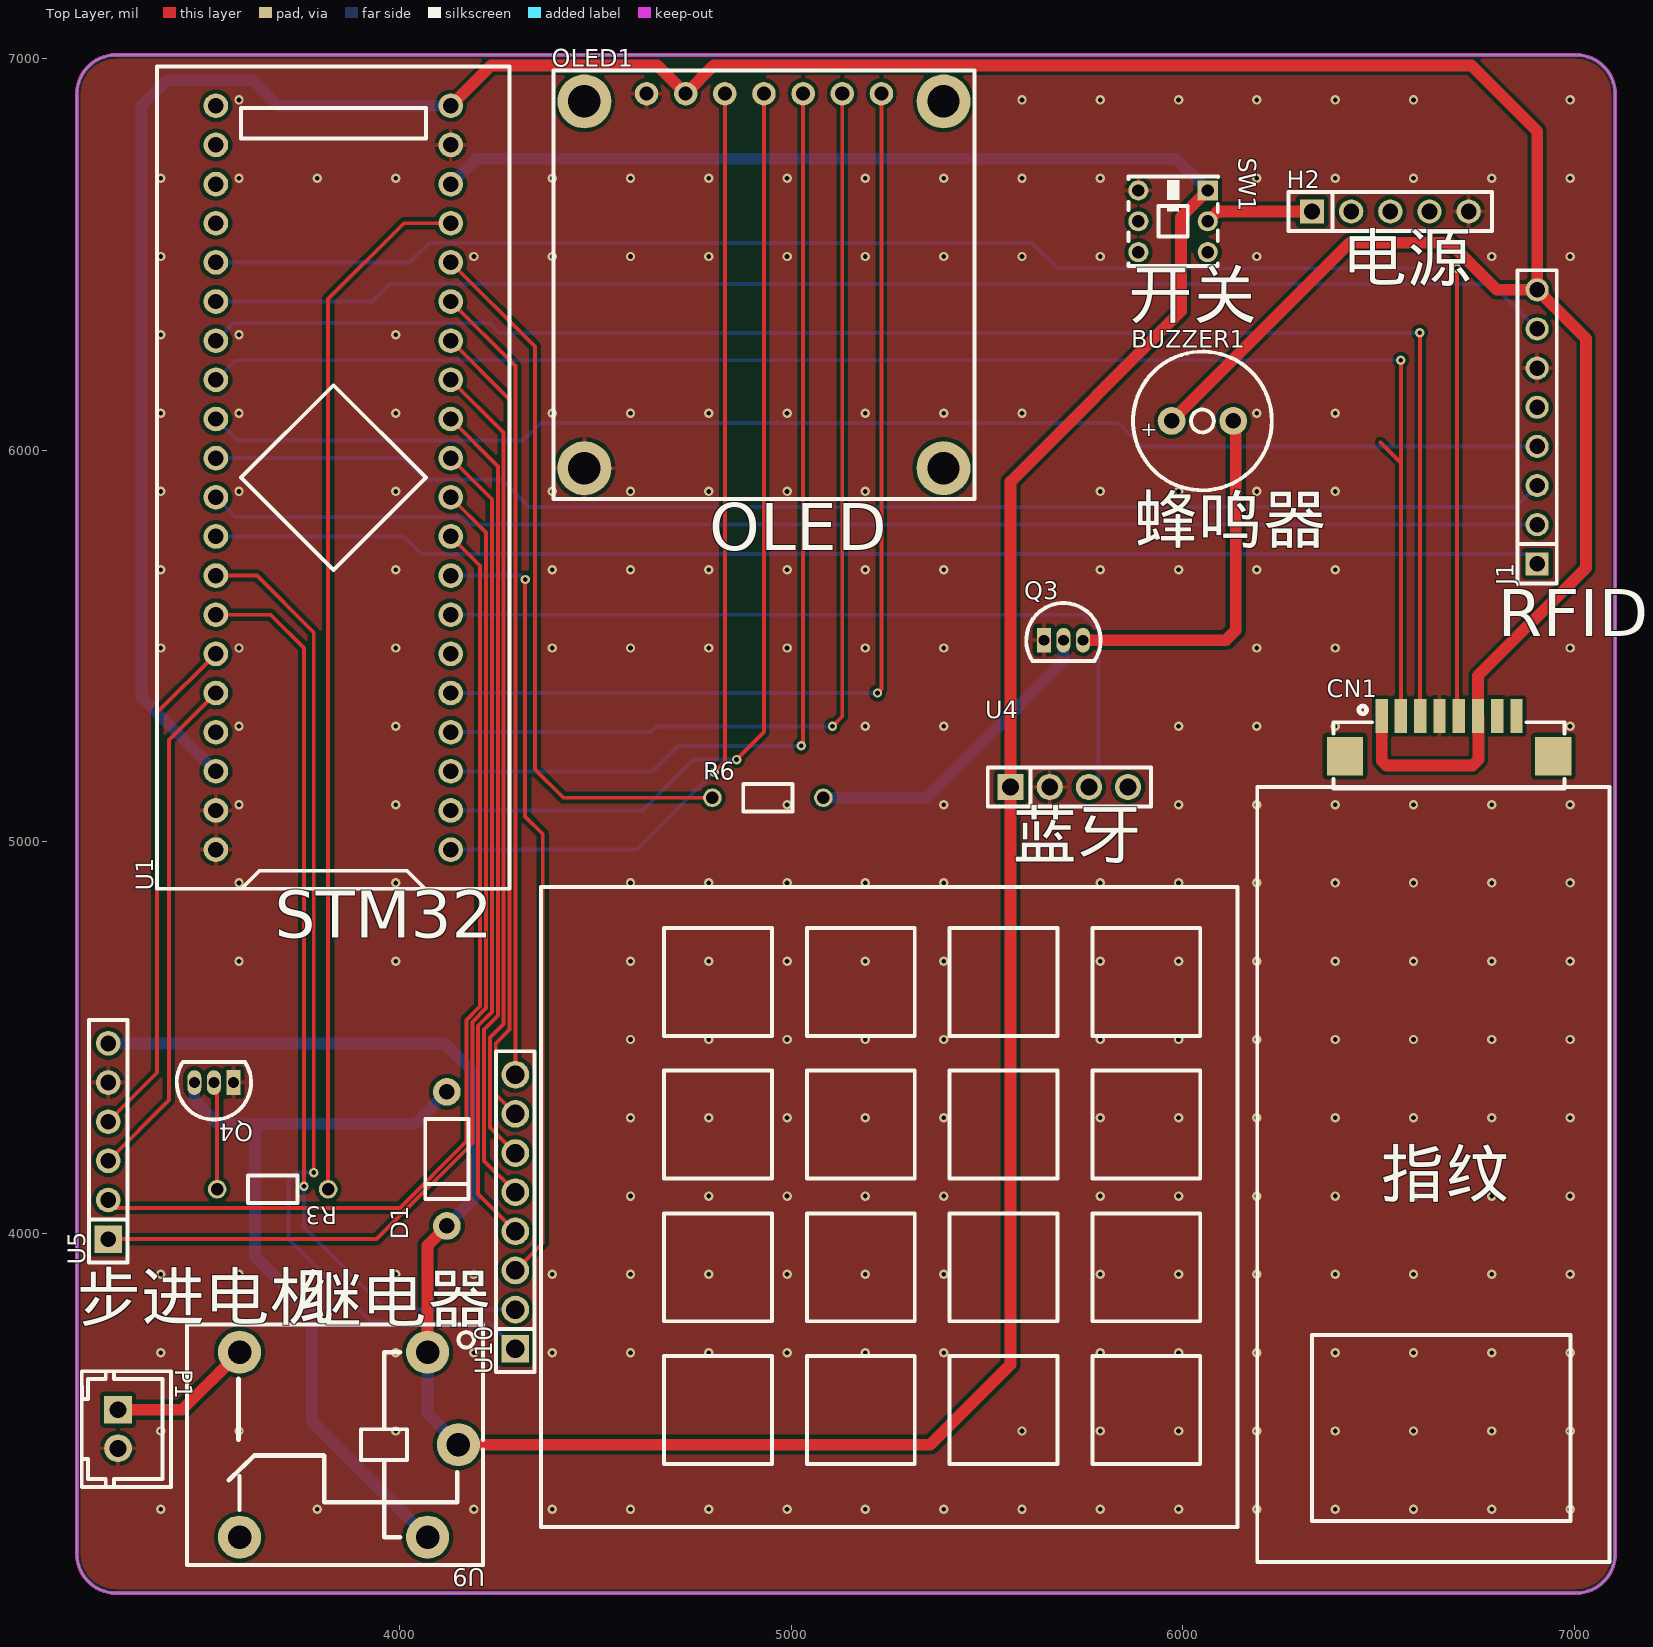
[diagram p0: Top Layer view]
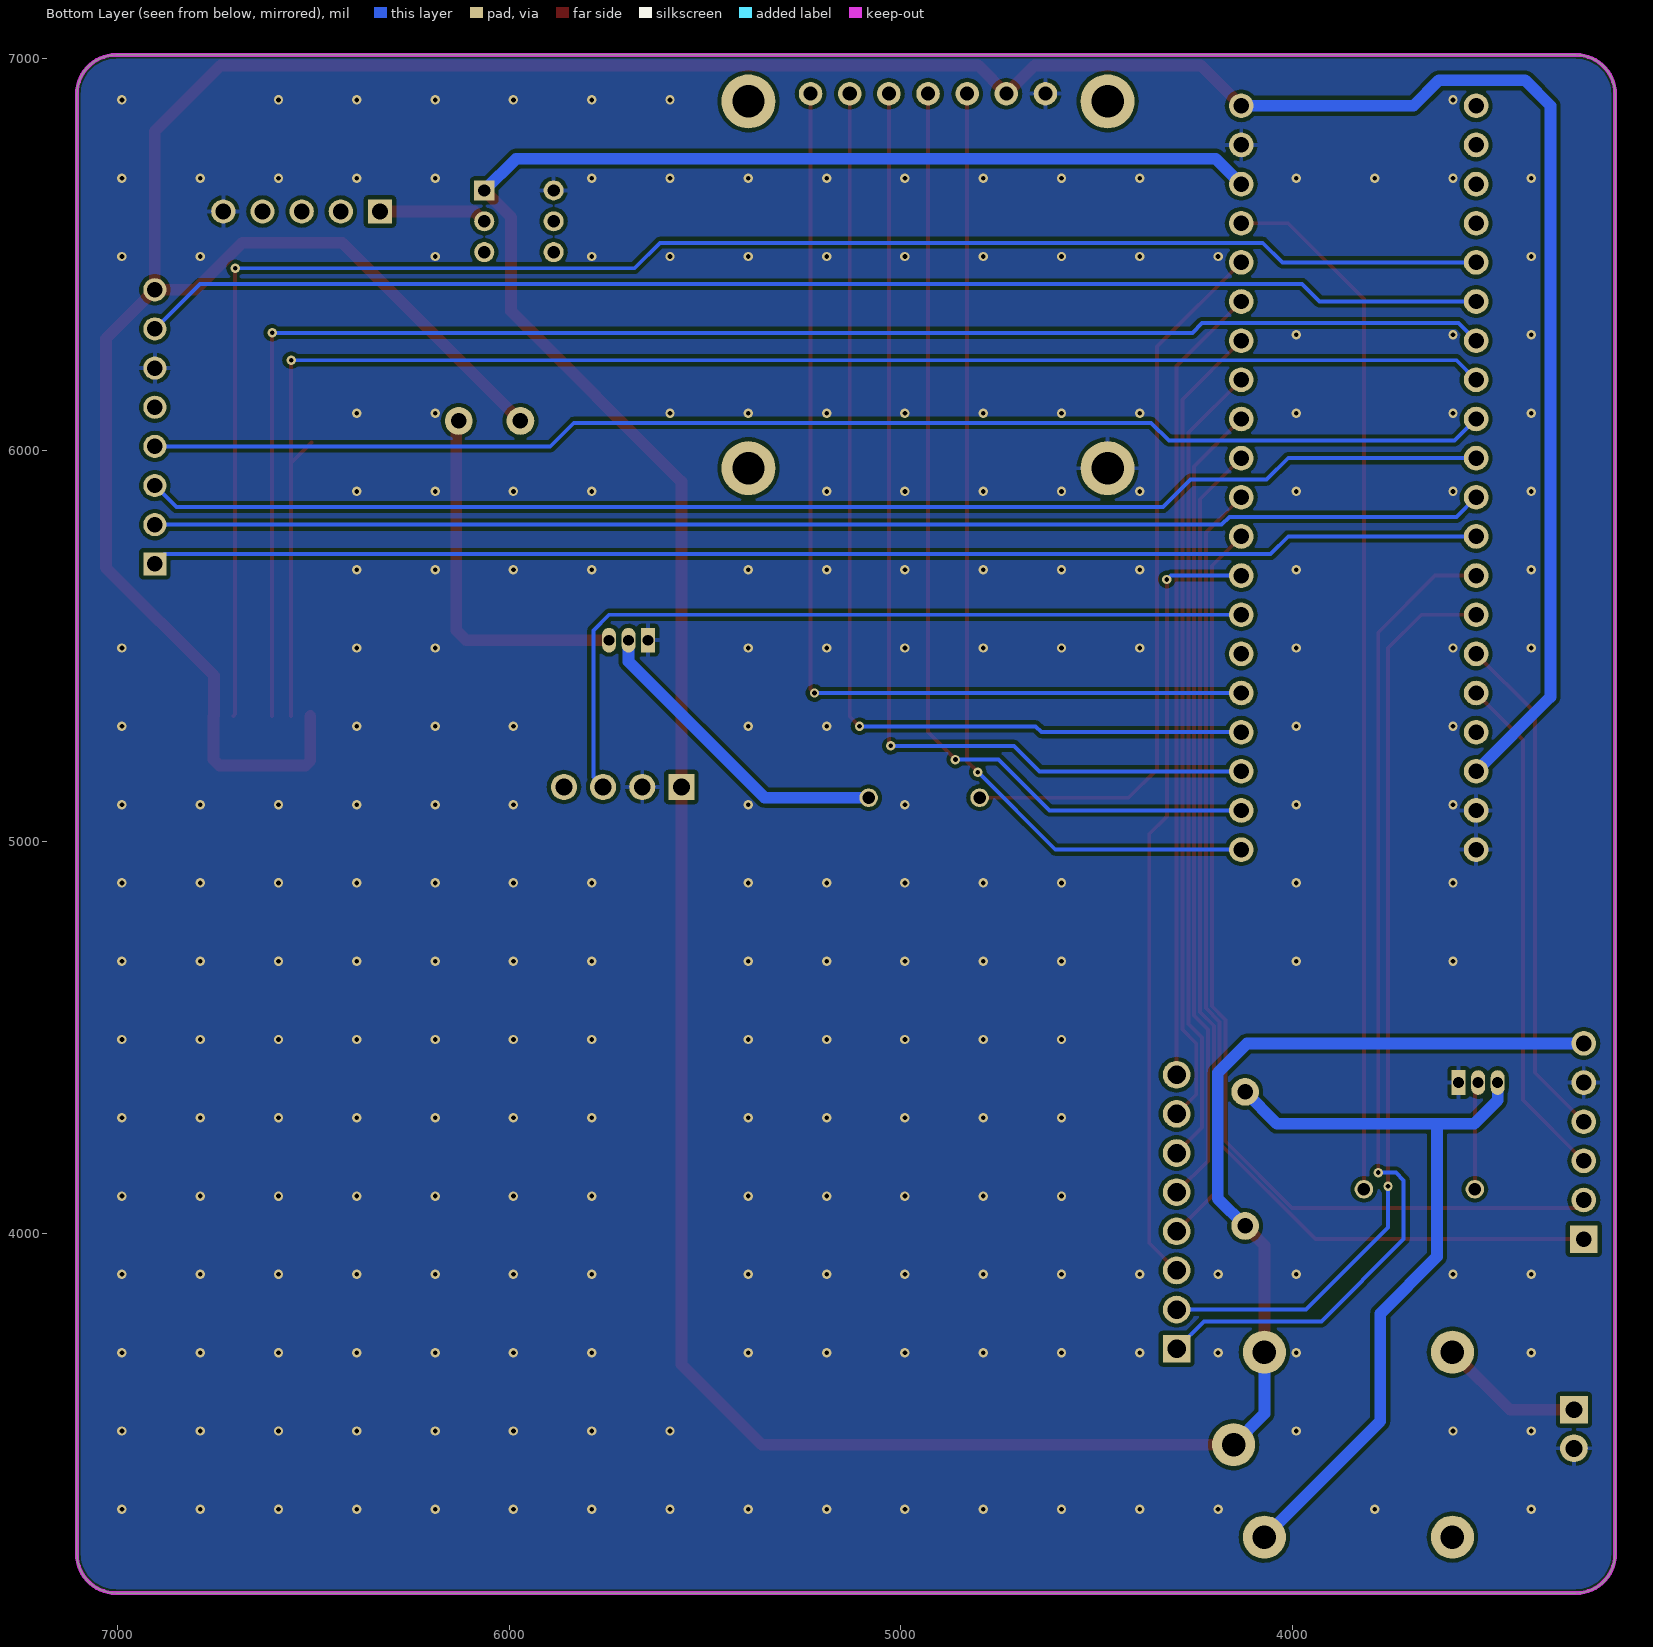
[diagram p1: Bottom Layer view, seen from below]
# Altium PCB MISC51826.pcbdoc
Units mil, origin at the board's own origin, x right, y up, seen from the top; angles counter-clockwise.
Board outline 3929.13 x 3929.13 mil, 2 copper layers (Top Layer, Bottom Layer), stack 62.206 mil thick; 17 components, 39 nets, 119 pads, 243 vias.

## Layer stack, top to bottom
Top Solder Mask Layer: solder mask 0.394, Dk 3.3
Top Layer: signal copper 1.379
Dielectric1: surface 59.449, FR4, Dk 4.5
Bottom Layer: signal copper 1.378
Bottom Solder Mask Layer: solder mask 0.394, Dk 3.3

## Board outline
3275,7010 ccw(c3275,6910) 3175,6910 3175,3180.87 ccw(c3275,3180.87) 3275,3080.87 7004.13,3080.87 ccw(c7004.13,3180.87) 7104.13,3180.87 7104.13,6910 ccw(c7004.13,6910) 7004.13,7010

## Design rules (kind name [scope] priority, off if disabled: settings)
BoardOutlineClearance copperThickness2oz_1 [All] p2 off: genericclearance=7.99 ignorepadtopadclearanceinfootprint=FALSE except(0: Arc-SplitContinuation Track-SplitContinuation SMDPad-SplitContinuation THPad-SplitContinuation Via-SplitContinuation Fill-SplitContinuation Region-SplitContinuation Poly-SplitContinuation Text-SplitContinuation Hole-SplitContinuation; 5.98: Arc-CutoutEdge SMDPad-CutoutEdge THPad-CutoutEdge Via-CutoutEdge Fill-CutoutEdge Region-CutoutEdge Text-CutoutEdge; 6.93: Hole-OutlineEdge Hole-CutoutEdge; 10: Poly-OutlineEdge Poly-CutoutEdge; 11.81: Arc-OutlineEdge Track-OutlineEdge SMDPad-OutlineEdge THPad-OutlineEdge Via-OutlineEdge Fill-OutlineEdge Region-OutlineEdge Text-OutlineEdge Track-CutoutEdge)
BoardOutlineClearance copperThickness1oz_1 [All] p4: genericclearance=4.02 ignorepadtopadclearanceinfootprint=FALSE except(0: Arc-SplitContinuation Track-SplitContinuation SMDPad-SplitContinuation THPad-SplitContinuation Via-SplitContinuation Fill-SplitContinuation Region-SplitContinuation Poly-SplitContinuation Text-SplitContinuation Hole-SplitContinuation; 6: SMDPad-CutoutEdge THPad-CutoutEdge Via-CutoutEdge Fill-CutoutEdge Region-CutoutEdge Text-CutoutEdge; 6.93: Hole-OutlineEdge Hole-CutoutEdge; 10: Poly-OutlineEdge Poly-CutoutEdge; 11.8: Arc-OutlineEdge Track-OutlineEdge SMDPad-OutlineEdge THPad-OutlineEdge Via-OutlineEdge Fill-OutlineEdge Region-OutlineEdge Text-OutlineEdge; 11.81: Arc-CutoutEdge Track-CutoutEdge)
Clearance copperThickness2oz [All] p1 off: gap=7.99 ignorepadtopadclearanceinfootprint=FALSE except(5.98: SMDPad-Track SMDPad-SMDPad THPad-Track SMDPad-THPad THPad-THPad Track-Via SMDPad-Via THPad-Via Via-Via Fill-Track Region-Track Fill-SMDPad Region-SMDPad Fill-THPad Region-THPad Fill-Via Region-Via Fill-Fill Fill-Region Region-Region Arc-Track Arc-SMDPad Arc-THPad Arc-Via Fill-Arc Region-Arc Arc-Arc Text-Track SMDPad-Text Text-THPad Text-Via Fill-Text Region-Text Arc-Text Text-Text; 6.93: Hole-Track Hole-SMDPad Hole-THPad Hole-Via Fill-Hole Region-Hole Hole-Arc Hole-Text; 10: Poly-Track Poly-SMDPad Poly-THPad Poly-Via Poly-Fill Poly-Region Poly-Poly Poly-Arc Poly-Text Poly-Hole)
Clearance copperThickness1oz [All] p3: gap=4.02 ignorepadtopadclearanceinfootprint=FALSE except(5.98: SMDPad-Track SMDPad-SMDPad THPad-Track SMDPad-THPad THPad-THPad Track-Via SMDPad-Via THPad-Via Via-Via Fill-Track Region-Track Fill-SMDPad Region-SMDPad Fill-THPad Region-THPad Fill-Via Region-Via Fill-Fill Fill-Region Region-Region; 6: Arc-Track Arc-SMDPad Arc-THPad Arc-Via Fill-Arc Region-Arc Arc-Arc Text-Track SMDPad-Text Text-THPad Text-Via Fill-Text Region-Text Arc-Text Text-Text; 6.93: Hole-Track Hole-SMDPad Hole-THPad Hole-Via Fill-Hole Region-Hole Hole-Arc Hole-Text; 10: Poly-Track Poly-SMDPad Poly-THPad Poly-Via Poly-Fill Poly-Region Poly-Poly Poly-Arc Poly-Text Poly-Hole)
DiffPairsRouting differentialPair [All] p1: maxlimit=6 minlimit=6 mostfreqgap=6 toplayer_minwidth=5 toplayer_prefwidth=10 toplayer_maxwidth=100 toplayer_mingap=6 toplayer_prefgap=6 toplayer_maxgap=6 bottomlayer_minwidth=5 bottomlayer_prefwidth=10 bottomlayer_maxwidth=100 bottomlayer_mingap=6 bottomlayer_prefgap=6 bottomlayer_maxgap=6 maxuncoupledlength=10
HoleToHoleClearance otherClearance [All] p1: gap=11.81 allowstackedmicrovias=TRUE
Length netLength [All] p1: minlimit=0 maxlimit=0
MatchedLengths netLengthTolerance [All] p1: tolerance=1000
PasteMaskExpansion pasteMaskExpansion [All] p1: expansion=0
PlaneConnect innerPlane [All] p1: planeconnectstyle=Relief reliefexpansion=20 reliefentries=4 reliefconductorwidth=10 reliefairgap=10
PolygonConnect copperRegion [(InNet('GND'))] p1: connectstyle=Relief reliefconductorwidth=10 reliefentries=4 polygonreliefangle="90 Angle" airgapwidth=10 via.connectstyle=Relief via.reliefconductorwidth=10 via.reliefentries=4 via.polygonreliefangle="90 Angle" via.airgapwidth=10
RoutingVias viaSize [All] p1: holewidth=12.01 width=24.02 viastyle="Through Hole" minholewidth=11.81 minwidth=19.68 maxholewidth=248.03 maxwidth=393.7
SolderMaskExpansion solderMaskExpansion [IsVia] p1: expansion=-1000 istentingtop=TRUE
SolderMaskExpansion solderMaskExpansion [All] p2: expansion=2 istentingtop=FALSE
Width copperThickness2oz_2 [All] p1 off: maxlimit=100 minlimit=8 preferedwidth=10
Width copperThickness1oz_2 [All] p2: maxlimit=100 minlimit=5 preferedwidth=10

## Components (designator, comment, footprint, x,y, rotation, side; value= is the part's Value field where it differs from the comment)
BUZZER1 "2.7kHz" BUZ-TH_BD9.0-P4.00-D0.6-FD 6050,6075 r0 top
CN1 "AS608" AS608 6680,5270 r0 top
D1 "" DO_1N4007 4120,4190 r90 top
H2 "" HDR-TH_5P-P2.54-V-F 6530,6610 r0 top
J1 "" HDR-TH_8P-P2.54-V-M 6905,6060 r90 top
OLED1 "" 0.96OLED 4930,6970 r0 top
P1 "WAFER-XH254Z-2A" CONN-TH_2P-P2.50_XH-2A_3045048 3280,3500 r270 top
Q3 "" S8050_TO_92 5695,5515 r0 top
Q4 "" S8050_TO_92 3525,4385 r180 top
R3 "1K" Res_1/8W 3675,4115 r180 top
R6 "1K" Res_1/8W 4940,5110 r0 top
SW1 "5.8 WSPT" SW-TH_6P-L5.8-W5.8-P2.00-LS4.5-TL_K8-5851E-L1 5975,6585 r270 top
U1 "LCKFB-DKX-STM32F103C8T6" CONN-TH_L53.3-W22.9_STM32F103C8T6-CARD 3830,5930 r90 top
U4 "" HDR-TH_4P-P2.54-V-F 5710,5140 r0 top
U5 "" HDR-TH_6P-P2.54-V-F 3255,4235 r90 top
U9 "SRD-12VDC-SL-C" RELAY-TH_SRD-XXVDC-XL-C 3870,3460 r180 top
U10 "" HDR-TH_8P-P2.54-V-F-1 4295,4055 r90 top

## Footprints (in the part's own frame and the unit in brackets; to place one, negate y for a bottom-side part, rotate by r counter-clockwise, add the part's x,y. Pads: shape width x height; smd on the part's side, far side on the other; paste and mask are expansions set on the pad)
0.96OLED [mm]
  round 3.5 hole 2.1: 0(-11.65,-2) 1(-11.65,-25.8) 8(11.65,-2) 9(11.65,-25.8)
  round 1.524 hole 0.914: 1(-7.62,-1.5) 2(-5.08,-1.5) 3(-2.54,-1.5) 4(0,-1.5) 5(2.54,-1.5) 6(5.08,-1.5) 7(7.62,-1.5)
  silkscreen extent -13.65,-27.8 13.65,0
AS608 [mm]
  rect 0.8x2.2 smd paste+0 mask+0.05: 1(-4.375,1.3) 2(-3.125,1.3) 3(-1.875,1.3) 4(-0.625,1.3) 5(0.625,1.3) 6(1.875,1.3) 7(3.125,1.3) 8(4.375,1.3)
  rect 2.35x2.5 smd paste+0 mask+0.05: 9(-6.755,-1.3) 10(6.755,-1.3)
  silkscreen extent -7.5,-3.4 7.5,1.95
BUZ-TH_BD9.0-P4.00-D0.6-FD [mm]
  round 1.8 hole 1: 1(-2,0) 2(2,0)
  silkscreen extent -4.5,-4.5 4.5,4.5
CONN-TH_2P-P2.50_XH-2A_3045048 [mm]
  rect 1.8x1.8 hole 1.1 paste+0 mask+0.05: 1(-1.25,0)
  round 1.8 hole 1.1 paste+0 mask+0.05: 2(1.25,0)
  silkscreen extent -3.75,-2.35 3.75,3.45
CONN-TH_L53.3-W22.9_STM32F103C8T6-CARD [mm]
  round 1.6 hole 1: 1(-24.13,-7.62) 2(-21.59,-7.62) 3(-19.05,-7.62) 4(-16.51,-7.62) 5(-13.97,-7.62) 6(-11.43,-7.62) 7(-8.89,-7.62) 8(-6.35,-7.62) 9(-3.81,-7.62) 10(-1.27,-7.62) 11(1.27,-7.62) 12(3.81,-7.62) 13(6.35,-7.62) 14(8.89,-7.62) 15(11.43,-7.62) 16(13.97,-7.62) 17(16.51,-7.62) 18(19.05,-7.62) 19(21.59,-7.62) 20(24.13,-7.62) 21(24.13,7.62) 22(21.59,7.62) 23(19.05,7.62) 24(16.51,7.62) 25(13.97,7.62) 26(11.43,7.62) 27(8.89,7.62) 28(6.35,7.62) 29(3.81,7.62) 30(1.27,7.62) 31(-1.27,7.62) 32(-3.81,7.62) 33(-6.35,7.62) 34(-8.89,7.62) 35(-11.43,7.62) 36(-13.97,7.62) 37(-16.51,7.62) 38(-19.05,7.62) 39(-21.59,7.62) 40(-24.13,7.62)
  silkscreen extent -26.67,-11.43 26.67,11.43
DO_1N4007 [mm]
  round 1.8 hole 1 paste+0 mask+0.051: 1(-4.35,0) 2(4.35,0)
  silkscreen extent -2.6,-1.4 2.6,1.4
HDR-TH_4P-P2.54-V-F [mm]
  rect 1.7x1.7 hole 1.1: 1(-3.81,0)
  round 1.7 hole 1.1: 2(-1.27,0) 3(1.27,0) 4(3.81,0)
  silkscreen extent -5.29,-1.27 5.29,1.27
HDR-TH_5P-P2.54-V-F [mil]
  rect 62x62 hole 40.16: 1(-200,0)
  round 62 hole 40.16: 2(-100,0) 3(0,0) 4(100,0) 5(200,0)
  silkscreen extent -260,-50 260,50
HDR-TH_6P-P2.54-V-F [mm]
  rect 1.8x1.8 hole 1.02: 1(-6.35,0)
  round 1.6 hole 1.02: 2(-3.81,0) 3(-1.27,0) 4(1.27,0) 5(3.81,0) 6(6.35,0)
  silkscreen extent -7.87,-1.25 7.87,1.25
HDR-TH_8P-P2.54-V-F-1 [mm]
  rect 1.8x1.8 hole 1.2: 1(-8.89,0)
  round 1.8 hole 1.2: 2(-6.35,0) 3(-3.81,0) 4(-1.27,0) 5(1.27,0) 6(3.81,0) 7(6.35,0) 8(8.89,0)
  silkscreen extent -10.41,-1.25 10.41,1.25
HDR-TH_8P-P2.54-V-M [mm]
  rect 1.5x1.5 hole 1: 1(-8.89,0)
  round 1.5 hole 1: 2(-6.35,0) 3(-3.81,0) 4(-1.27,0) 5(1.27,0) 6(3.81,0) 7(6.35,0) 8(8.89,0)
  silkscreen extent -10.16,-1.27 10.16,1.27
RELAY-TH_SRD-XXVDC-XL-C [mil]
  round 110 hole 60: 1(-200.79,-236.22) 2(279.53,-236.2) 3(279.53,236.2) 4(-200.79,236.22) 5(-279.53,0)
  silkscreen extent -342,-307 413,307
Res_1/8W [mil]
  round 47.2 hole 31.5 paste+0 mask+2: 1(-141.7,2.48) 2(141.7,2.48)
  silkscreen extent -63,-33 63,38
S8050_TO_92 [mil]
  rect 35.4x63 hole 27.6 paste+0 mask+2: 1(-50,0)
  oval 35.4x63 hole 27.6 paste+0 mask+2: 2(0,0) 3(50,0)
  silkscreen extent -95,-53 95,95
SW-TH_6P-L5.8-W5.8-P2.00-LS4.5-TL_K8-5851E-L1 [mm]
  rect 1.3x1.3 hole 0.8 paste+0 mask+0.05: 1(-2,2.25)
  round 1.3 hole 0.8 paste+0 mask+0.05: 2(0,2.25) 3(2,2.25) 4(-2,-2.25) 5(0,-2.25) 6(2,-2.25)
  silkscreen extent -2.9,-2.9 2.9,2.92

## Via types
v1: diameter 24.02, hole 12, Top Layer to Bottom Layer, 243 vias

## Nets (pads, with @x,y where several pads share a name; then routed paths per layer and width w, separated by ;. In a path a pad name is that pad's centre, name@x,y a point inside that pad or via, vN(x,y) a via of type N, cw(c..) or ccw(c..) an arc to the next point about the centre after c; other vN are vias at no path point)
$1N3: Q4.2 R3.2 | length 275.9
  Top Layer w10: Q4.2 3533.3,4376.7 R3.2
$1N6: D1.2 Q4.3 U9.4 | length 1977.3
  Bottom Layer w30: Q4.3 3475,4340 3535,4280 4038.74,4280 D1.2 ; 3630,4270 3630,3940 3775,3795 3775,3519.57 U9.4
$1N8: P1.1 U9.2 | length 371.4
  Top Layer w30: P1.1 3443.48,3549.21 U9.2
$1N34: H2.1 SW1.2 | length 276.8
  Top Layer w30: SW1.2 6088.59,6610 H2.1
$1N53: Q3.2 R6.2 | length 812.2
  Bottom Layer w30: R6.2 5347.48,5112.48 5695,5460 Q3.2
$1N55: BUZZER1.2 Q3.3 | length 937.9
  Top Layer w30: Q3.3 6110,5515 6135,5540 6135,6068.74 BUZZER1.2
$1N71: U1.37
+5V: D1.1 SW1.1 U1.18 U4.1 U5.6 U9.1 U9.5 | length 8694.9
  Top Layer w30: U9.1 4070.79,3969.53 D1.1 ; U9.5 5355,3460 5560,3665 U4.1 5560,5920 5995,6355 5995,6595.15 SW1.1
  Bottom Layer w30: U5.6 4115,4485 4190,4410 4190,4088.74 D1.1 ; U9.1 4070.79,3538.74 U9.5 ; U1.18 4195,6745 5982.32,6745 SW1.1
BEEP: R6.1 U1.16 | length 1867.4
  Top Layer w10: U1.16 4345,6265 4345,5185 4417.52,5112.48 R6.1
GND: CN1.4 H2.5 J1.6 OLED1.1 P1.2 Q3.1 Q4.1 SW1.4 U1.19 U1.39 U1.40 U4.2 U5.5
  other v1: 3389.1,3294.97 3789.1,3294.97 4189.1,3294.97 4389.1,3294.97 4589.1,3294.97 4789.1,3294.97 4989.1,3294.97 5189.1,3294.97 5389.1,3294.97 5589.1,3294.97 5789.1,3294.97 5989.1,3294.97 6189.1,3294.97 6389.1,3294.97 6589.1,3294.97 6789.1,3294.97 6989.1,3294.97 3389.1,3494.97 3589.1,3494.97 3989.1,3494.97 5589.1,3494.97 5789.1,3494.97 5989.1,3494.97 6189.1,3494.97 6389.1,3494.97 6589.1,3494.97 6789.1,3494.97 6989.1,3494.97 3389.1,3694.97 3989.1,3694.97 4189.1,3694.97 4389.1,3694.97 4589.1,3694.97 4789.1,3694.97 4989.1,3694.97 5189.1,3694.97 5389.1,3694.97 5789.1,3694.97 5989.1,3694.97 6189.1,3694.97 6389.1,3694.97 6589.1,3694.97 6789.1,3694.97 6989.1,3694.97 3389.1,3894.97 3589.1,3894.97 3989.1,3894.97 4189.1,3894.97 4389.1,3894.97 4589.1,3894.97 4789.1,3894.97 4989.1,3894.97 5189.1,3894.97 5389.1,3894.97 5789.1,3894.97 5989.1,3894.97 6189.1,3894.97 6389.1,3894.97 6589.1,3894.97 6789.1,3894.97 6989.1,3894.97 4589.1,4094.97 4789.1,4094.97 4989.1,4094.97 5189.1,4094.97 5389.1,4094.97 5789.1,4094.97 5989.1,4094.97 6189.1,4094.97 6389.1,4094.97 6589.1,4094.97 6789.1,4094.97 6989.1,4094.97 4589.1,4294.97 4789.1,4294.97 4989.1,4294.97 5189.1,4294.97 5389.1,4294.97 5789.1,4294.97 5989.1,4294.97 6189.1,4294.97 6389.1,4294.97 6589.1,4294.97 6789.1,4294.97 6989.1,4294.97 4589.1,4494.97 4789.1,4494.97 4989.1,4494.97 5189.1,4494.97 5389.1,4494.97 5789.1,4494.97 5989.1,4494.97 6189.1,4494.97 6389.1,4494.97 6589.1,4494.97 6789.1,4494.97 6989.1,4494.97 3589.1,4694.97 3989.1,4694.97 4589.1,4694.97 4789.1,4694.97 4989.1,4694.97 5189.1,4694.97 5389.1,4694.97 5789.1,4694.97 5989.1,4694.97 6189.1,4694.97 6389.1,4694.97 6589.1,4694.97 6789.1,4694.97 6989.1,4694.97 3589.1,4894.97 3989.1,4894.97 4589.1,4894.97 4789.1,4894.97 4989.1,4894.97 5189.1,4894.97 5389.1,4894.97 5789.1,4894.97 5989.1,4894.97 6189.1,4894.97 6389.1,4894.97 6589.1,4894.97 6789.1,4894.97 6989.1,4894.97 3589.1,5094.97 3989.1,5094.97 4989.1,5094.97 5389.1,5094.97 5989.1,5094.97 6189.1,5094.97 6389.1,5094.97 6589.1,5094.97 6789.1,5094.97 6989.1,5094.97 3589.1,5294.97 3989.1,5294.97 5189.1,5294.97 5389.1,5294.97 5989.1,5294.97 6189.1,5294.97 6389.1,5294.97 6989.1,5294.97 3389.1,5494.97 3589.1,5494.97 3989.1,5494.97 4389.1,5494.97 4589.1,5494.97 4789.1,5494.97 4989.1,5494.97 5189.1,5494.97 5389.1,5494.97 6189.1,5494.97 6389.1,5494.97 6989.1,5494.97 3389.1,5694.97 3989.1,5694.97 4389.1,5694.97 4589.1,5694.97 4789.1,5694.97 4989.1,5694.97 5189.1,5694.97 5389.1,5694.97 5789.1,5694.97 5989.1,5694.97 6189.1,5694.97 6389.1,5694.97 3389.1,5894.97 3589.1,5894.97 3989.1,5894.97 4389.1,5894.97 4589.1,5894.97 4789.1,5894.97 4989.1,5894.97 5189.1,5894.97 5789.1,5894.97 5989.1,5894.97 6189.1,5894.97 6389.1,5894.97 3389.1,6094.97 3589.1,6094.97 3989.1,6094.97 4389.1,6094.97 4589.1,6094.97 4789.1,6094.97 4989.1,6094.97 5189.1,6094.97 5389.1,6094.97 5589.1,6094.97 6189.1,6094.97 6389.1,6094.97 3389.1,6294.97 3589.1,6294.97 3989.1,6294.97 3389.1,6494.97 4189.1,6494.97 4389.1,6494.97 4589.1,6494.97 4789.1,6494.97 4989.1,6494.97 5189.1,6494.97 5389.1,6494.97 5589.1,6494.97 5789.1,6494.97 6189.1,6494.97 6789.1,6494.97 6989.1,6494.97 3389.1,6694.97 3589.1,6694.97 3789.1,6694.97 3989.1,6694.97 4389.1,6694.97 4589.1,6694.97 4789.1,6694.97 4989.1,6694.97 5189.1,6694.97 5389.1,6694.97 5589.1,6694.97 5789.1,6694.97 6189.1,6694.97 6389.1,6694.97 6589.1,6694.97 6789.1,6694.97 6989.1,6694.97 3589.1,6894.97 5589.1,6894.97 5789.1,6894.97 5989.1,6894.97 6189.1,6894.97 6389.1,6894.97 6589.1,6894.97 6989.1,6894.97
IN1: U1.10 U5.1 | length 2733.3
  Top Layer w10: U5.1 3940,3985 4185,4230 4185,4540 4220,4575 4220,5790 U1.10
IN2: U1.9 U5.2 | length 2584.3
  Top Layer w10: U5.2 3275,4065 4000,4065 4170,4235 4170,4545 4205,4580 4205,5705 U1.9
IN3: U1.36 U5.3 | length 1308.9
  Top Layer w10: U5.3 3410,4340 3410,5260 U1.36
IN4: U1.35 U5.4 | length 1308.9
  Top Layer w10: U5.4 3380,4410 3380,5330 U1.35
JDQ: R3.1 U1.17 | length 2667.5
  Top Layer w10: R3.1 3816.7,6386.7 4010,6580 U1.17
MFR_MISO: J1.4 U1.29 | length 3441.3
  Bottom Layer w10: U1.29 3585,6025 4315,6025 4360,6070 5835,6070 5895,6010 J1.4
MFR_MOSI: J1.3 U1.30 | length 3449.6
  Bottom Layer w10: U1.30 4010,5980 4065,5925 4260,5925 4330,5855 6850,5855 J1.3
MFR_RST: J1.7 U1.26 | length 3441.3
  Bottom Layer w10: U1.26 3930,6380 3975,6425 6790,6425 J1.7
MFR_SCK: J1.2 U1.31 | length 3404
  Bottom Layer w10: U1.31 3580,5830 4160,5830 4180,5810 J1.2
MFR_SDA: J1.1 U1.32 | length 3404
  Bottom Layer w10: U1.32 4010,5780 4055,5735 6880,5735 J1.1
OLED_CS: OLED1.7 U1.5 | length 2625.1
  Top Layer w10: v1(5220,5380) 5230,5390 OLED1.7
  Bottom Layer w10: U1.5 v1(5220,5380)
OLED_D0: OLED1.3 U1.1 | length 2499.1
  Top Layer w10: v1(4802.88,5177.88) 4830,5205 OLED1.3
  Bottom Layer w10: U1.1 4605,4980 v1(4802.88,5177.88)
OLED_D1: OLED1.4 U1.2 | length 2513.8
  Top Layer w10: v1(4860,5210) 4930,5280 OLED1.4
  Bottom Layer w10: U1.2 4620,5080 4750,5210 v1(4860,5210)
OLED_DC: OLED1.6 U1.4 | length 2607.5
  Top Layer w10: v1(5105,5295) 5130,5320 OLED1.6
  Bottom Layer w10: U1.4 4640,5280 4655,5295 v1(5105,5295)
OLED_RES: OLED1.5 U1.3 | length 2589.9
  Top Layer w10: v1(5025,5245) 5030,5250 OLED1.5
  Bottom Layer w10: U1.3 4645,5180 4710,5245 v1(5025,5245)
SW1: U1.33 U10.1 | length 2609.3
  Top Layer w10: U1.33 3635,5680 3780,5535 v1(3780,4155)
  Bottom Layer w10: v1(3780,4155) 3735,4155 3715,4135 3715,3985 3925,3775 4225,3775 U10.1
SW2: U1.34 U10.2 | length 2367.2
  Top Layer w10: U1.34 3670,5580 3755,5495 v1(3755,4120)
  Bottom Layer w10: v1(3755,4120) 3755,4015 3965,3805 U10.2
SW3: U1.8 U10.3 | length 2006.8
  Top Layer w10: U10.3 4365,3975 4365,5020 4320,5065 v1(4320,5670)
  Bottom Layer w10: U1.8 4310,5680 v1(4320,5670)
SW4: U1.11 U10.4 | length 2072.3
  Top Layer w10: U1.11 4235,5875 4235,4565 4200,4530 4200,4100 U10.4
SW5: U1.12 U10.5 | length 2073.2
  Top Layer w10: U1.12 4250.98,5959.02 4250.98,4555.98 4215,4520 4215,4185 U10.5
SW6: U1.13 U10.6 | length 2072.3
  Top Layer w10: U1.13 4265,6045 4265,4535 4230,4500 4230,4270 U10.6
SW7: U1.14 U10.7 | length 2072.3
  Top Layer w10: U1.14 4280,6130 4280,4520 4245,4485 4245,4355 U10.7
SW8: U1.15 U10.8 | length 2043.3
  Top Layer w10: U1.15 4295,6215 U10.8
TOUCH: CN1.5 U1.25 | length 4363.4
  Top Layer w10: v1(6700,6465) 6700,5325.78 CN1.5
  Bottom Layer w10: U1.25 4025,6480 4075,6530 5615,6530 5680,6465 v1(6700,6465)
UART1_RX: U1.7 U4.3 | length 2081.9
  Bottom Layer w10: U1.7 5745,5580 5785,5540 5785,5165 U4.3
UART2_RX: CN1.2 U1.28 | length 4030
  Top Layer w10: 6505,6020 6556.97,5968.03 ; CN1.2 6556.97,5968.03 ; v1(6556.97,6230) 6556.97,5968.03
  Bottom Layer w10: U1.28 3580,6230 v1(6556.97,6230)
UART2_TX: CN1.3 U1.27 | length 4083.3
  Top Layer w10: v1(6605,6300) 6606.18,6298.82 CN1.3
  Bottom Layer w10: U1.27 3575,6325 4230,6325 4255,6300 v1(6605,6300)
UATR1_TX: U1.6
VCC: BUZZER1.1 CN1.1 CN1.6 J1.8 OLED1.2 U1.20 U1.38 | length 8885.9
  Top Layer w30: U1.20 4233.2,6983.2 4657.74,6983.2 OLED1.2 4802.26,6983.2 6736.8,6983.2 6905,6815 J1.8 ; BUZZER1.1 6426.26,6530 6681.66,6530 6801.66,6410 J1.8 ; CN1.1 6507.76,5207.24 6520,5195 6740,5195 6755,5210 6755,5319.99 CN1.6 6753.81,5423.81 7030,5700 7030,6285 J1.8
  Bottom Layer w30: U1.38 3340,5370 3340,6880 3405,6945 3625,6945 3690,6880 U1.20
pads on no net: CN1.7 CN1.8 CN1.9 CN1.10 H2.2 H2.3 H2.4 J1.5 OLED1.0 OLED1.8 OLED1.9 SW1.3 SW1.5 SW1.6 U1.21 U1.22 U1.23 U1.24 U4.4 U9.3

## Polygon pours and split planes (outlines as drawn)
GND on Top Layer (solid, remove dead copper, pour order 0): 3120,7020 3120,3040 7120,3040 7120,7020
GND on Bottom Layer (solid, remove dead copper, pour order 2): 3120,7025 3120,3050 7115,3050 7115,7025

## Keep-outs
Board Outline Layer:
  the board outline again, w10

## Silkscreen, mask and mechanical layers (free items; w line width, h text height)
Top Silkscreen Layer:
  lines w10: 4360,3250 4360,4885 6140,4885 6140,3250 4360,3250 ; 4675,3410.59 4675,3686.18 4950.59,3686.18 4950.59,3410.59 4675,3410.59 ; 4675,3775.2 4675,4050.79 4950.59,4050.79 4950.59,3775.2 4675,3775.2 ; 4675,4139.8 4675,4415.39 4950.59,4415.39 4950.59,4139.8 4675,4139.8 ; 4675,4504.41 4675,4780 4950.59,4780 4950.59,4504.41 4675,4504.41 ; 5039.61,3410.59 5039.61,3686.18 5315.2,3686.18 5315.2,3410.59 5039.61,3410.59 ; 5039.61,3775.2 5039.61,4050.79 5315.2,4050.79 5315.2,3775.2 5039.61,3775.2 ; 5039.61,4139.8 5039.61,4415.39 5315.2,4415.39 5315.2,4139.8 5039.61,4139.8 ; 5039.61,4504.41 5039.61,4780 5315.2,4780 5315.2,4504.41 5039.61,4504.41 ; 5404.21,3410.59 5404.21,3686.18 5679.8,3686.18 5679.8,3410.59 5404.21,3410.59 ; 5404.21,3775.2 5404.21,4050.79 5679.8,4050.79 5679.8,3775.2 5404.21,3775.2 ; 5404.21,4139.8 5404.21,4415.39 5679.8,4415.39 5679.8,4139.8 5404.21,4139.8 ; 5404.21,4504.41 5404.21,4780 5679.8,4780 5679.8,4504.41 5404.21,4504.41 ; 5768.82,3410.59 5768.82,3686.18 6044.41,3686.18 6044.41,3410.59 5768.82,3410.59 ; 5768.82,3775.2 5768.82,4050.79 6044.41,4050.79 6044.41,3775.2 5768.82,3775.2 ; 5768.82,4139.8 5768.82,4415.39 6044.41,4415.39 6044.41,4139.8 5768.82,4139.8 ; 5768.82,4504.41 5768.82,4780 6044.41,4780 6044.41,4504.41 5768.82,4504.41 ; 6190,3160 6190,5140 7090,5140 7090,3160 6190,3160 ; 6330,3265 6330,3740 6990,3740 6990,3265 6330,3265
  text "电源" at 6410,6435 h120
  text "开关" at 5860,6340 h120
  text "蜂鸣器" at 5875,5765 h120
  text "OLED" at 4790,5745 h120
  text "RFID" at 6805,5525 h120
  text "蓝牙" at 5565,4960 h120
  text "STM32" at 3680,4755 h120
  text "指纹" at 6505,4095 h120
  text "步进电机" at 3175,3780 h120
  text "继电器" at 3740,3775 h120